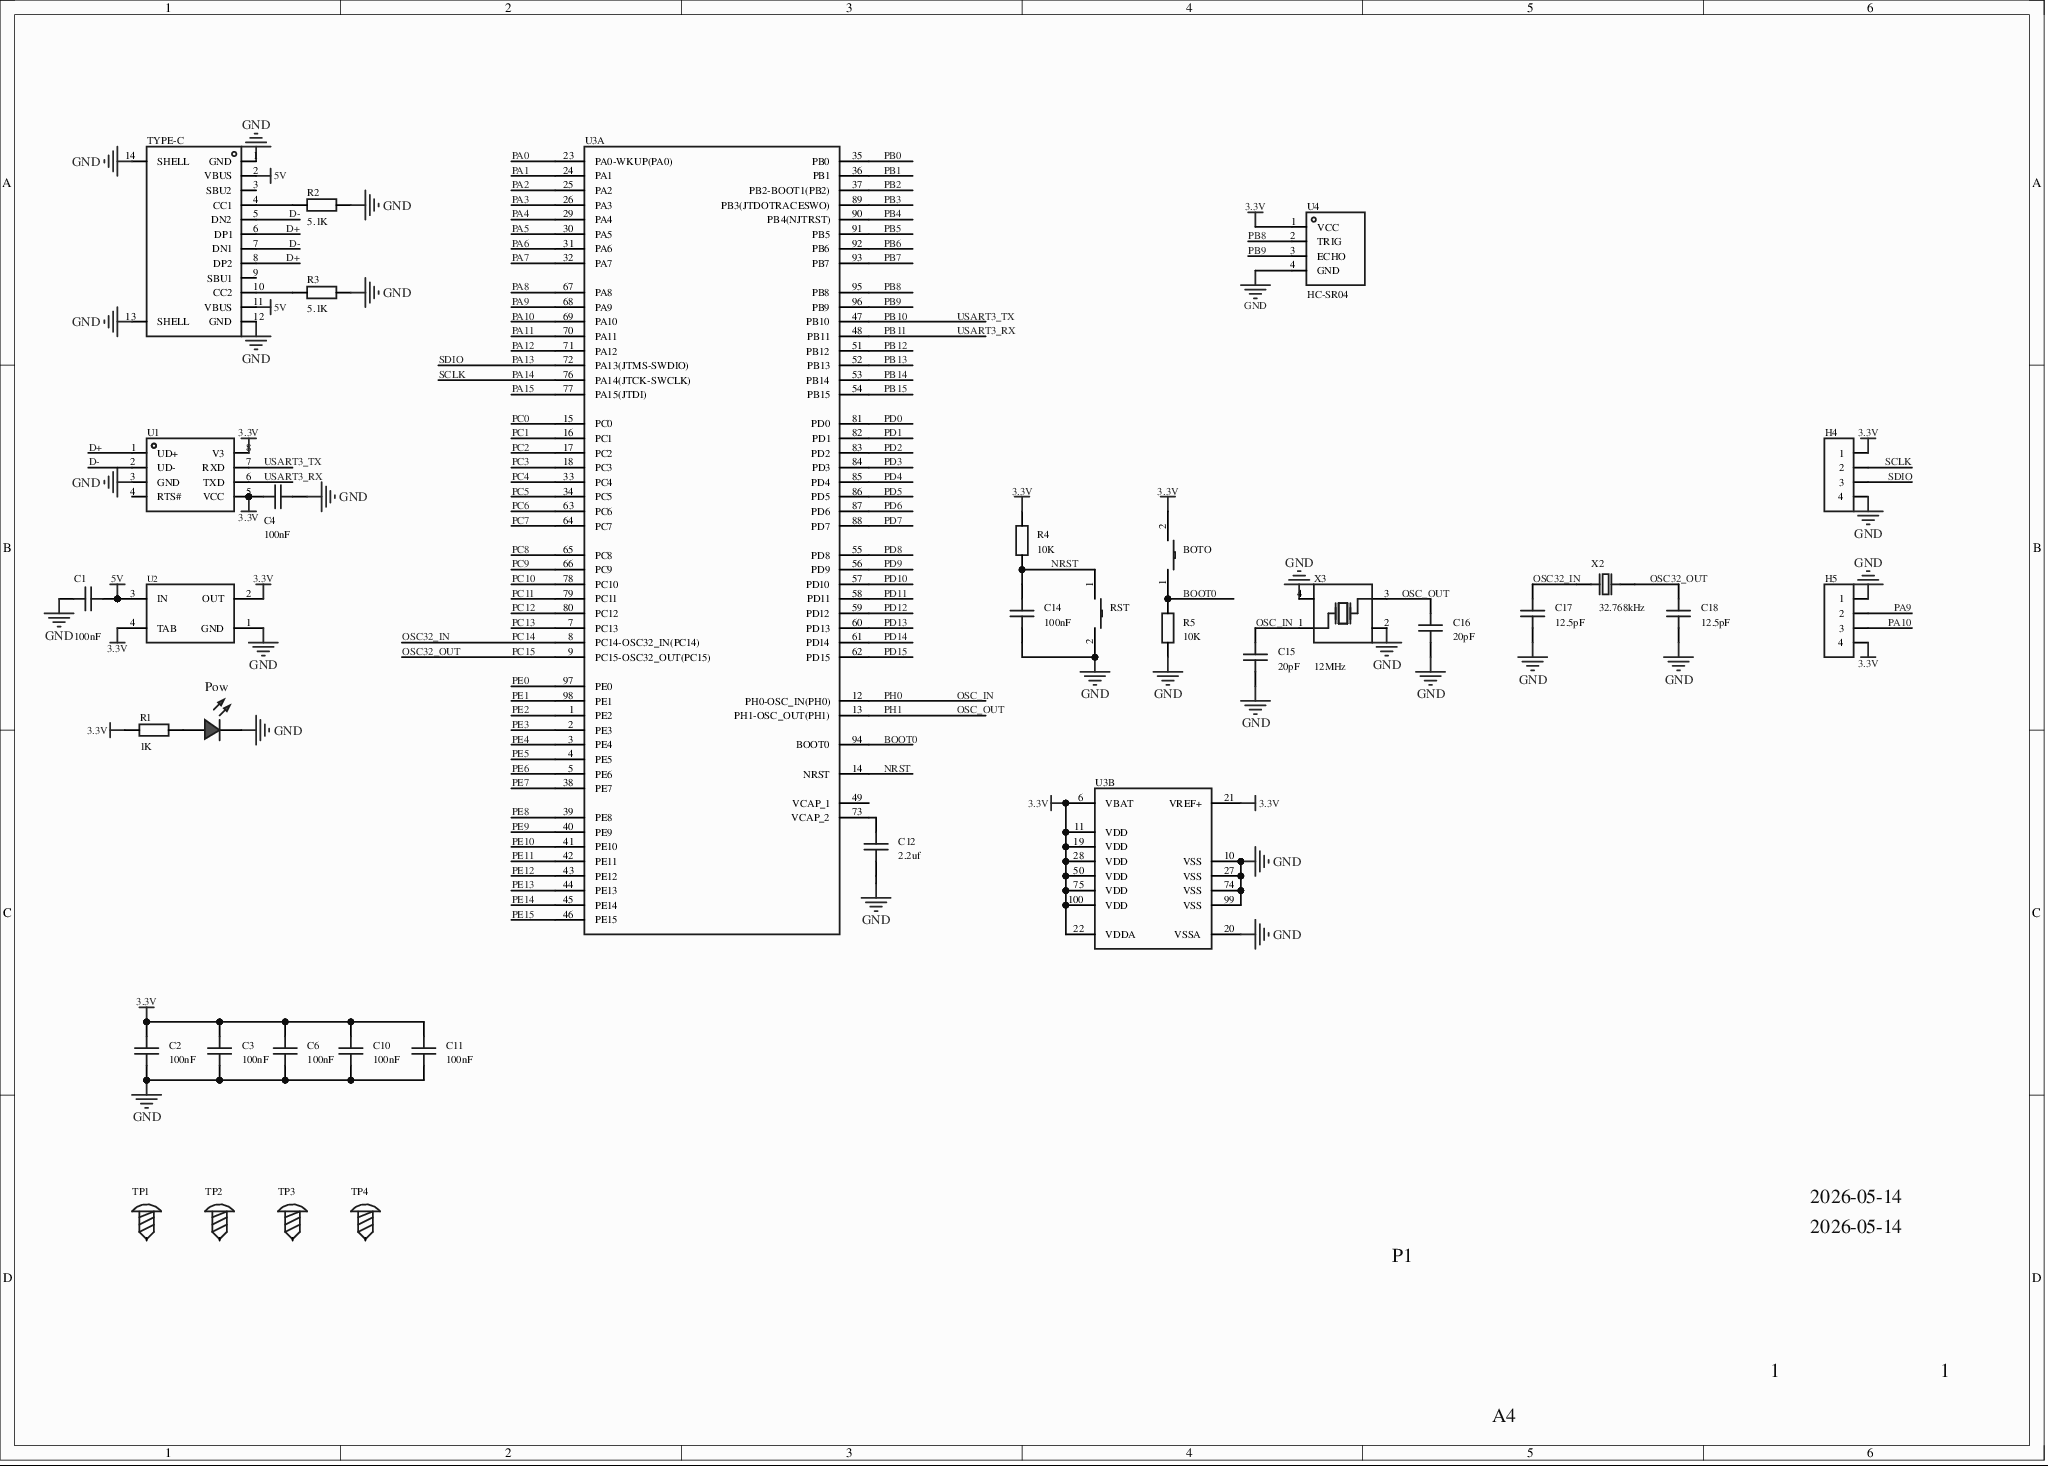
[diagram p0: MISC61235-3.schdoc]
# Altium project MISC61235-2.PrjPcb
1 sheet, 34 parts. Net scope: global (net labels, ports and power ports of the same name join across sheets).
Board file: MISC61235.pcbdoc

## Sheet MISC61235-3.schdoc
size 355 x 254 mm; Version: V1.0; @Project Name: MISC61235; @Page Count: 1; @Update Date: 2026-05-14; @Create Date: 2026-05-14; @Schematic Name: MISC61235; @Page No: 1

### Parts
BOTO  TS-1101-C-W  [SW-SMD_L6.0-W3.3-LS8.0]  (value not drawn)
C1  value 100nF  [C0603]  (hidden comment: CAP_0603)
C2  value 100nF  [C0603]  (hidden comment: CAP_0603)
C3  value 100nF  [C0603]  (hidden comment: CAP_0603)
C4  value 100nF  [C0603]  (hidden comment: CAP_0603)
C6  value 100nF  [C0603]  (hidden comment: CAP_0603)
C10  value 100nF  [C0603]  (hidden comment: CAP_0603)
C11  value 100nF  [C0603]  (hidden comment: CAP_0603)
C12  value 2.2uf  [C0603]  (hidden comment: CAP_0603)
C14  value 100nF  [C0603]  (hidden comment: CAP_0603)
C15  value 20pF  [C0603]  (hidden comment: CAP_0603)
C16  value 20pF  [C0603]  (hidden comment: CAP_0603)
C17  value 12.5pF  [C0603]  (hidden comment: CAP_0603)
C18  value 12.5pF  [C0603]  (hidden comment: CAP_0603)
H4  Side-solder 1X4 pin header  [侧焊1X4排针]  (value not drawn)
H5  Side-solder 1X4 pin header  [侧焊1X4排针]  (value not drawn)
Pow  LED_0603-R  [LED_0603]  (value not drawn)
R1  value 1K  [R0603]  (hidden comment: Res_0603)
R2  value 5.1K  [R0603]  (hidden comment: Res_0603)
R3  value 5.1K  [R0603]  (hidden comment: Res_0603)
R4  value 10K  [R0603]  (hidden comment: Res_0603)
R5  value 10K  [R0603]  (hidden comment: Res_0603)
RST  TS-1101-C-W  [SW-SMD_L6.0-W3.3-LS8.0]  (value not drawn)
TP1  M3 screw  [M3螺丝]  (value not drawn)
TP2  M3 screw  [M3螺丝]  (value not drawn)
TP3  M3 screw  [M3螺丝]  (value not drawn)
TP4  M3 screw  [M3螺丝]  (value not drawn)
TYPE-C  TYPE-C 16PIN 2MD(073)  [USB-C-SMD_TYPE-C-6PIN-2MD-073]  (value not drawn)
U1  CH340N  [SOP-8_L4.9-W3.9-P1.27-LS6.0-BL]  (value not drawn)
U2  LM1117IMPX-3.3/NOPB  [SOT-223_L6.5-W3.5-P2.30-LS7.0-BR]  (value not drawn)
U3  (no value)  [LQFP-100_L14.0-W14.0-P0.50-LS16.0-BL]  (parts A,B of 2)
U4  HC-SR04  [TH_HC-SR04V]
X2  value 32.768kHz  [FC-135R_L3.2-W1.5]  (hidden comment: Q13FC1350000400)
X3  value 12MHz  [OSC-SMD_4P-L3.2-W2.5-BL]  (hidden comment: X322512MSB4SI)

### Nets
3.3V: BOTO.2 C2.2 C3.2 C4.1 C6.2 C10.2 C11.2 H4.1 H5.4 R1.1 R4.2 U1.5(VCC) U1.8(V3) U2.2(OUT) U2.4(TAB) U3.6(VBAT) U3.11(VDD) U3.19(VDD) U3.21(VREF+) U3.22(VDDA) U3.28(VDD) U3.50(VDD) U3.75(VDD) U3.100(VDD) U4.1(VCC)
5V: C1.2 TYPE-C.2(VBUS) TYPE-C.11(VBUS) U2.3(IN)
GND: C1.1 C2.1 C3.1 C4.2 C6.1 C10.1 C11.1 C12.2 C14.1 C15.1 C16.1 C17.1 C18.1 H4.4 H5.1 Pow.1(C) R2.1 R3.1 R5.1 RST.2 TYPE-C.1(GND) TYPE-C.12(GND) TYPE-C.13(SHELL) TYPE-C.14(SHELL) U1.3(GND) U2.1(GND) U3.10(VSS) U3.20(VSSA) U3.27(VSS) U3.74(VSS) U3.99(VSS) U4.4(GND) X3.2(GND) X3.4(GND)
BOOT0: BOTO.1 R5.2 U3.94(BOOT0)
D+: TYPE-C.6(DP1) TYPE-C.8(DP2) U1.1(UD+)
D-: TYPE-C.5(DN2) TYPE-C.7(DN1) U1.2(UD-)
NRST: C14.2 R4.1 RST.1 U3.14(NRST)
OSC32_IN: C17.2 U3.8(PC14-OSC32_IN(PC14)) X2.1  [also labelled PC14]
OSC32_OUT: C18.2 U3.9(PC15-OSC32_OUT(PC15)) X2.2  [also labelled PC15]
OSC_IN: C15.2 U3.12(PH0-OSC_IN(PH0)) X3.1(OSC1)  [also labelled PH0]
OSC_OUT: C16.2 U3.13(PH1-OSC_OUT(PH1)) X3.3(OSC2)  [also labelled PH1]
PA0: U3.23(PA0-WKUP(PA0))
PA1: U3.24(PA1)
PA2: U3.25(PA2)
PA3: U3.26(PA3)
PA4: U3.29(PA4)
PA5: U3.30(PA5)
PA6: U3.31(PA6)
PA7: U3.32(PA7)
PA8: U3.67(PA8)
PA9: H5.2 U3.68(PA9)
PA10: H5.3 U3.69(PA10)
PA11: U3.70(PA11)
PA12: U3.71(PA12)
PA13: H4.3 U3.72(PA13(JTMS-SWDIO))  [also labelled SDIO]
PA14: H4.2 U3.76(PA14(JTCK-SWCLK))  [also labelled SCLK]
PA15: U3.77(PA15(JTDI))
PB0: U3.35(PB0)
PB1: U3.36(PB1)
PB2: U3.37(PB2-BOOT1(PB2))
PB3: U3.89(PB3(JTDOTRACESWO))
PB4: U3.90(PB4(NJTRST))
PB5: U3.91(PB5)
PB6: U3.92(PB6)
PB7: U3.93(PB7)
PB8: U3.95(PB8) U4.2(TRIG)
PB9: U3.96(PB9) U4.3(ECHO)
PB10: U1.7(RXD) U3.47(PB10)  [also labelled USART3_TX]
PB11: U1.6(TXD) U3.48(PB11)  [also labelled USART3_RX]
PB12: U3.51(PB12)
PB13: U3.52(PB13)
PB14: U3.53(PB14)
PB15: U3.54(PB15)
PC0: U3.15(PC0)
PC1: U3.16(PC1)
PC2: U3.17(PC2)
PC3: U3.18(PC3)
PC4: U3.33(PC4)
PC5: U3.34(PC5)
PC6: U3.63(PC6)
PC7: U3.64(PC7)
PC8: U3.65(PC8)
PC9: U3.66(PC9)
PC10: U3.78(PC10)
PC11: U3.79(PC11)
PC12: U3.80(PC12)
PC13: U3.7(PC13)
PD0: U3.81(PD0)
PD1: U3.82(PD1)
PD2: U3.83(PD2)
PD3: U3.84(PD3)
PD4: U3.85(PD4)
PD5: U3.86(PD5)
PD6: U3.87(PD6)
PD7: U3.88(PD7)
PD8: U3.55(PD8)
PD9: U3.56(PD9)
PD10: U3.57(PD10)
PD11: U3.58(PD11)
PD12: U3.59(PD12)
PD13: U3.60(PD13)
PD14: U3.61(PD14)
PD15: U3.62(PD15)
PE0: U3.97(PE0)
PE1: U3.98(PE1)
PE2: U3.1(PE2)
PE3: U3.2(PE3)
PE4: U3.3(PE4)
PE5: U3.4(PE5)
PE6: U3.5(PE6)
PE7: U3.38(PE7)
PE8: U3.39(PE8)
PE9: U3.40(PE9)
PE10: U3.41(PE10)
PE11: U3.42(PE11)
PE12: U3.43(PE12)
PE13: U3.44(PE13)
PE14: U3.45(PE14)
PE15: U3.46(PE15)
NetC12_1: C12.1 U3.73(VCAP_2)
NetPow_2: Pow.2(A) R1.2
NetR2_2: R2.2 TYPE-C.4(CC1)
NetR3_2: R3.2 TYPE-C.10(CC2)

Not connected (* = marked no-connect by the designer): TP1 1*; TP2 1*; TP3 1*; TP4 1*; TYPE-C 3(SBU2)* 9(SBU1)*; U1 4(RTS#)*; U3 49(VCAP_1)

### Notes on the sheet
- 2026-05-14
- P1
- A4
- 1

### Library data of the parts
BOTO RST = TS-1101-C-W: Contact current: 50mA; rated voltage (AC): -; rated voltage (DC): 12V; rated power: -; insulation resistance: -; circuit structure: SPST; mounting: SMD vertical; with lamp: no; actuating force: 260gf; mechanical life: 5万 cycles; with bracket: no;; Manufacturer: XKB Connectivity(中国星坤); AddInBom: yes; ModelId: b2f4ea9f0afc4b0786d53dba66ceb9e4; ModelName: SW-SMD_L6.0-W3.3-H5-LS8.0; ModelTransform: 314.96,129.921,0,0,0,0,0,0,0; Actuator Style: Rectangular button; Actuator/Cap Color: White with light green; With Lamp: None; Switch Length: 6mm; Switch Width: 3.6mm; Switch Height: 2.5mm; Symbol: TS-1101-C-W; Device: TS-1101-C-W; LCSC Part Name: 立贴 6*3.6*2.5mm 轻触开关 一型3*6*2.5有白ZD b拉伸白色带淡绿按键 卷装; SupplierPart: C318938; ManufacturerPart: TS-1101-C-W; Supplier Footprint: SMD; JLCPCB Part Class: Extended library; Datasheet: https://atta.szlcsc.com/upload/public/pdf/source/20200227/C318938_C2E53B1EEDE37D980A33616AC086DE53.pdf; Supplier: LCSC; ConvertToPcb: yes; FootprintName: SW-SMD_L6.0-W3.3-LS8.0; Contact Current: 50mA; Voltage Rating (AC): -; Voltage Rating (DC): 12V; Power Rating: -; Insulation Resistance: -; Circuit: SPST; Mounting Style: SMD vertical; Operating Force: 260gf; Mechanical Life: 5万 cycles; Operating Temperature: -30℃~+85℃; IP Rating: -; Pin Style: -; Diameter: -; Strike Gundam: No
C1-C4 C12 C14-C18 = CAP_0603: ConvertToPcb: yes; SymbolName: CapAcitance; ModelId: ac125912035d415993ca9572d50418b1; ModelName: C0603_L1.6-W0.8-H0.8; ModelTransform: 62.992,31.496,0,0,0,0,0,0,0; Device: CAP_0603; AddInBom: yes; Supplier Footprint: 0603; FootprintName: C0603
C6 C10 C11 = CAP_0603: Symbol: CapAcitance; ConvertToPcb: yes; ModelId: ac125912035d415993ca9572d50418b1; ModelName: C0603_L1.6-W0.8-H0.8; ModelTransform: 62.992,31.496,0,0,0,0,0,0,0; Device: CAP_0603; AddInBom: yes; Supplier Footprint: 0603; FootprintName: C0603
H4 H5 = 侧焊1X4排针: AddInBom: yes; Device: Side-solder 1X4 pin header; ConvertToPcb: yes; SymbolName: Side-solder 1X4 pin header; FootprintName: Side-solder 1X4 pin header
Pow = LED_0603-R: Symbol: LED_R; Convert to PCB: yes; 3D Model: dd8257b0d61a4cd7b68939a056e08095; 3D Model Transform: 58.72,29.4,22.03,0,0,0,0,0,0; ModelName: LED-0603_R; Device: LED_0603-R; Add into BOM: yes; Supplier Footprint: 0603; FootprintName: LED_0603
R1-R5 = Res_0603: Symbol: Resistor; ConvertToPcb: yes; ModelId: fc143cca1e79419f9cd78b61e9279f08; ModelTransform: 31.8897,63.7794,0,90,0,0,0,0,0; Device: Res_0603; AddInBom: yes; Supplier Footprint: 0603; FootprintName: R0603; ModelName: R0603
TP1-TP4 = M3螺丝: ConvertToPcb: yes; SymbolName: Screw hole; Device: M3 screw; AddInBom: yes; Supplier Footprint: 插件; FootprintName: M3 screw
TYPE-C = TYPE-C 16PIN 2MD(073): Connector type: Type-C; standard: -; gender: female; contact count: 16P; port count: 1; mounting: SMD horizontal; rated current - power: 5A; operating temperature: -25℃~+85℃;; Manufacturer: SHOU HAN(首韩); AddInBom: yes; ModelId: 3a41b9ec9b654a0fad4d118405ec6290; ModelTransform: 351.9678,298.4246,0,0,0,0,0,-47.244,-35.433; Number of Ports: 1; Symbol: TYPE-C 16PIN 2MD(073); Device: TYPE-C 16PIN 2MD(073); Supplier: LCSC; Supplier Part: C2765186; Manufacturer Part: TYPE-C 16PIN 2MD(073); JLCPCB Part Class: Extended Part; LCSC Part Name: Type-C 母 卧贴 带定位柱 不锈钢外壳 2次模顶; Supplier Footprint: SMD; Datasheet: https://atta.szlcsc.com/upload/public/pdf/source/20211123/39B17C16241EAC15C5E277BDA434118E.pdf; ConvertToPcb: yes; FootprintName: USB-C-SMD_TYPE-C-6PIN-2MD-073; ModelName: USB-C-SMD_TYPE-C-6PIN-2MD-073; Connector Type: Type-C; Standard: -; Gender: Female; Number of Contacts: 16P; Mounting Style: SMD horizontal; Current Rating - Power (Max): 5A; Operating Temperature Range: -25℃~+85℃
U1 = CH340N: Manufacturer: WCH(南京沁恒); Symbol: CH340N_C2977777; AddInBom: yes; ModelId: 75c24a7891ee4dd6bdac16a7163ff87e; ModelName: SOP-8_L4.9-W3.9-P1.27-LS6.0-BL-1; ModelTransform: 192.913,236.22,0,0,0,0,0,0,0; Device: CH340N; Supplier: LCSC; Supplier Part: C2977777; Manufacturer Part: CH340N; JLCPCB Part Class: Extended Part; LCSC Part Name: USB转串口芯片 CH340; Supplier Footprint: SOP-8; Datasheet: https://atta.szlcsc.com/upload/public/pdf/source/20230530/6E401E9554E9F5311886CC8B3F89B62E.pdf; ConvertToPcb: yes; FootprintName: SOP-8_L4.9-W3.9-P1.27-LS6.0-BL
U2 = LM1117IMPX-3.3/NOPB: Output type: fixed; output polarity: positive; max input voltage: 15V; output voltage: 3.3V; output current: 800mA; ripple rejection (PSRR): 75dB@(120Hz);; Manufacturer: TI(德州仪器); AddInBom: yes; ModelId: 925194bf9823436183a3e0b978a8d076; ModelName: SOT-223-4P_L6.5-W3.5-H1.6-LS7.0-P2.30; ModelTransform: 279.89794,255.905,0,180,0,0,0.0005,0.0005,0; Number of Outputs: 1; Dropout Voltage: 1.2V@(800mA); Quiescent Current (Ground Current): 5mA; Symbol: LM1117IMPX-3.3/NOPB; Device: LM1117IMPX-3.3/NOPB; Supplier: LCSC; Manufacturer Part: LM1117IMPX-3.3/NOPB; Supplier Part: C23984; JLCPCB Part Class: Extended library; LCSC Part Name: 输入20V 输出3.3V 800mA; Supplier Footprint: SOT-223; Datasheet: http://www.ti.com/cn/lit/gpn/lm1117; ConvertToPcb: yes; FootprintName: SOT-223_L6.5-W3.5-P2.30-LS7.0-BR; Output Type: Fixed; Output Polarity: Positive; Maximum Input Voltage: 15V; Output Voltage: 3.3V; Output Current: 800mA; Power Supply Rejection Ratio (PSRR): 75dB@(120Hz); Operating Temperature: -40℃~+125℃
U3 = STM32F407VET6: CPU core: ARM Cortex-M4; max CPU frequency: 168MHz; operating voltage: 1.8V~3.6V; internal oscillator: yes; program FLASH: 512K@x8bit; total RAM: 192KB; EEPROM/data FLASH: -; GPIO ports: 82; ADC (units/channels/bits): 1@x16ch/12bit; DAC (units/channels/bits): 1@x2ch/12bit; peripherals/functions/protocol stacks: undervoltage detection/reset; DMA; LCD driver; watchdog; POR; PWM; operating temperature: -40℃~+85℃;; Manufacturer: ST(意法半导体); 3D Model: 469e6cc70557486dbd01fd12ff814964; 3D Model Transform: 629.92,629.92,0,0,0,0,0,0,0; GPIO Ports Number: 82; ModelName: LQFP-100_L14.0-W14.0-H1.4-LS16.0-P0.50; Symbol: STM32F407VET6; Device: STM32F407VET6; LCSC Part Name: ARM Cortex-M4 168MHz 闪存：512K@x8bit RAM：192KB; Supplier Part: C28730; Manufacturer Part: STM32F407VET6; Supplier Footprint: LQFP-100(14x14); JLCPCB Part Class: Extended library; Datasheet: https://atta.szlcsc.com/upload/public/pdf/source/20140322/1457707027869.pdf; Supplier: LCSC; CPU Core: ARM Cortex-M4; Maximum Frequency: 168MHz; Supply Voltage Range: 1.8V~3.6V; Internal Oscillator: Yes; Program FLASH Size: 512K@x8bit; RAM Size: 192KB; EEPROM/Data FLASH Size: -; ADC (Units/Channels/bits): 1@x16ch/12bit; DAC (Units/Channels/bits): 1@x2ch/12bit; Peripherals / Functions / Protocol Stacks: Undervoltage detection/reset; DMA; LCD driver; watchdog; POR; PWM; Operating Temperature Range: -40℃~+85℃; AddInBom: yes; ConvertToPcb: yes; FootprintName: LQFP-100_L14.0-W14.0-P0.50-LS16.0-BL
U4 = HC-SR04: Manufacturer: Universal Microelectronics; AddInBom: yes; Symbol: HC-SR04; Device: HC-SR04; LCSC Part Name: HC-SR04; SupplierPart: C19857336; ManufacturerPart: HC-SR04; Supplier Footprint: -; JLCPCB Part Class: Extended Part; Datasheet: https://item.szlcsc.com/datasheet/HC-SR04/21184790.html; Supplier: LCSC; ConvertToPcb: yes; FootprintName: TH_HC-SR04V
X2 = Q13FC1350000400: Frequency: 32.768kHz; frequency tolerance: ±20ppm; load capacitance: 12.5pF;; Manufacturer: EPSON(爱普生); AddInBom: yes; ModelId: b5334dc599ac49d68fb741bd067a525d; ModelName: SMD-3215_2P_L3.2-W1.5-H0.8; ModelTransform: 125.984,59.055,0,0,0,0,0,0,0; Crystal Type: SMD passive crystal; Equivalent Series Resistance (ESR): 70kΩ; Symbol: Q13FC1350000400; Device: Q13FC1350000400; LCSC Part Name: 32.768kHz ±20ppm 12.5pF; SupplierPart: C32346; ManufacturerPart: Q13FC1350000400; Supplier Footprint: SMD3215-2P; JLCPCB Part Class: Basic library; Datasheet: https://atta.szlcsc.com/upload/public/pdf/source/20190108/C32346_746D6B07EAF90824457A96480007685F.pdf; Supplier: LCSC; ConvertToPcb: yes; FootprintName: FC-135R_L3.2-W1.5; Frequency Tolerance: ±20ppm; Load Capacitance: 12.5pF; Operating Temperature: -40℃~+85℃
X3 = X322512MSB4SI: Crystal type: SMD crystal; frequency: 12MHz; frequency tolerance (room temp): ±10ppm; external load capacitance: 20pF; frequency stability (full temp): ±30ppm;; Manufacturer: YXC(扬兴晶振); AddInBom: yes; ModelId: ae22b8d143894765bc8100c37cb6356f; ModelName: OSC-SMD_4P-L3.2-W2.5-H1.0; ModelTransform: 125.984,98.425,0,0,0,0,0,0,0; Symbol: X322512MSB4SI; Device: X322512MSB4SI; LCSC Part Name: 12MHz ±10ppm 20pF; SupplierPart: C9002; ManufacturerPart: X322512MSB4SI; Supplier Footprint: SMD3225-4P; JLCPCB Part Class: Basic library; Datasheet: https://atta.szlcsc.com/upload/public/pdf/source/20210329/C112971_1F611BDC486E193C1706F6D8EB5AA189.pdf; Supplier: LCSC; ConvertToPcb: yes; FootprintName: OSC-SMD_4P-L3.2-W2.5-BL; Crystal Type: SMD crystal; Normal temperature Frequency Tolerance: ±10ppm; External load capacitor: 20pF; Frequency Stability(Full temperature range): ±30ppm; Operating Temperature: -40℃~+85℃